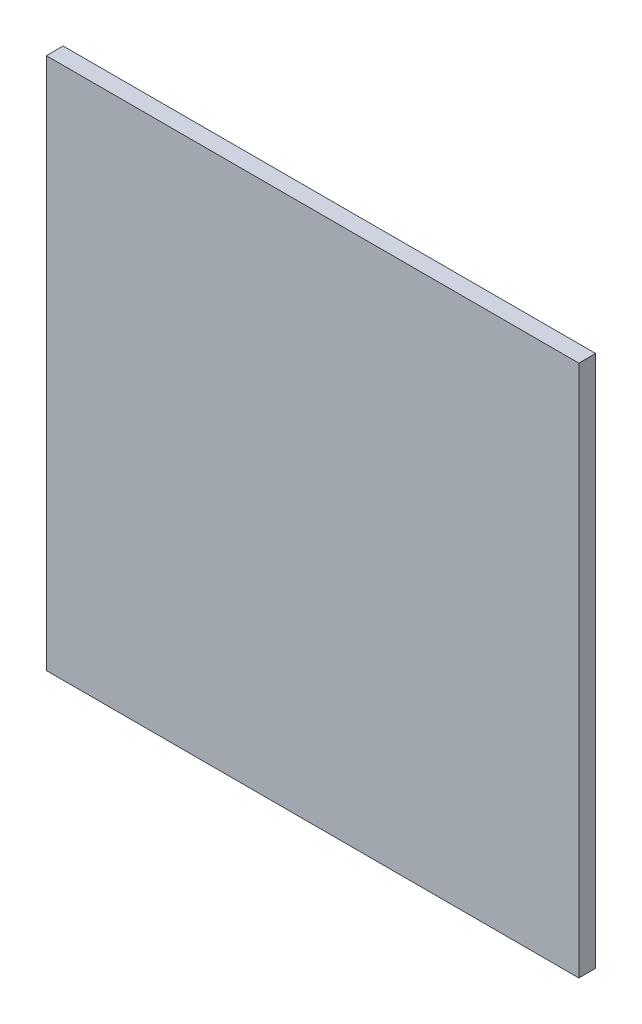
SolidWorks part; units mm, degrees
material "普通碳钢"
ref_plane "Front Plane" through (0, 0, 0) normal (0, 0, 1) x (1, 0, 0)
ref_plane "Top Plane" through (0, 0, 0) normal (0, 1, 0) x (1, 0, 0)
ref_plane "Right Plane" through (0, 0, 0) normal (1, 0, 0) x (0, 0, -1)
sketch "Sketch1" plane through (0, 0, 0) normal (0, 0, 1) x (1, 0, 0)
  line L1 (-127, 127) -> (127, 127)
  line L2 (-127, 127) -> (-127, -127)
  line L3 (-127, -127) -> (127, -127)
  line L4 (127, 127) -> (127, -127)
  dimension "D1" = 254
  dimension "D2" = 127
  dimension "D3" = 254
  dimension "D4" = 127
extrude "Boss-Extrude1" add sketch "Sketch1" along normal mid plane 8
